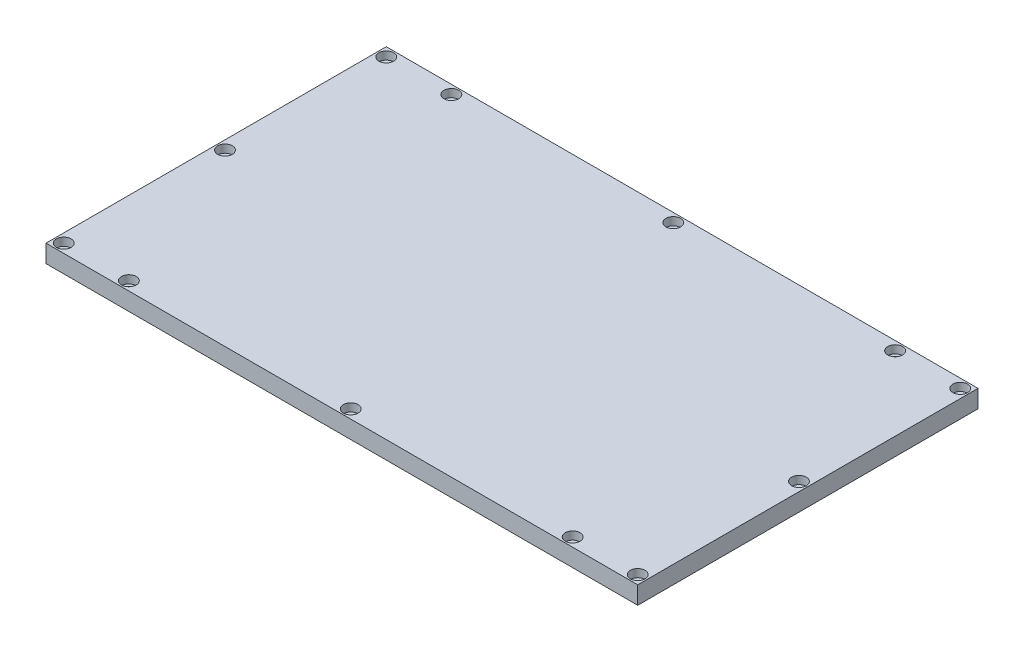
SolidWorks part; units mm, degrees
material "国产6061 "
ref_plane "Front Plane" through (0, 0, 0) normal (0, 0, 1) x (1, 0, 0)
ref_plane "Top Plane" through (0, 0, 0) normal (0, 1, 0) x (1, 0, 0)
ref_plane "Right Plane" through (0, 0, 0) normal (1, 0, 0) x (0, 0, -1)
sketch "Sketch1" plane through (0, 0, 0) normal (0, 1, 0) x (1, 0, 0)
  line L1 (-200, 115) -> (200, 115)
  line L2 (-200, 115) -> (-200, -115)
  line L3 (-200, -115) -> (200, -115)
  line L4 (200, 115) -> (200, -115)
  line L5 (-200, 115) -> (200, -115) construction
  line L6 (-200, -115) -> (200, 115) construction
  point P0 (0, 0)
  dimension "D1" = 400
  dimension "D2" = 230
extrude "Boss-Extrude1" add sketch "Sketch1" along normal blind 12
hole_wizard "CBORE for M5 Hex Socket Head Cap Screw1" positions "Sketch2" profile "Sketch3" counterbore size "M5" standard "ISO"
sketch "Sketch2" plane through (0, 12, 0) normal (0, 1, 0) x (1, 0, 0)
  line L0 (200, 115) -> (-200, 115) construction
  line L1 (-200, 115) -> (-200, -115) construction
  line L2 (-200, -115) -> (200, -115) construction
  line L3 (200, -115) -> (200, 115) construction
  point P0 (-194, 109)
  point P2 (-150, 109)
  point P4 (150, 109)
  point P6 (194, 109)
  point P8 (194, 0)
  point P10 (194, -109)
  point P12 (150, -109)
  point P14 (-150, -109)
  point P16 (-194, -109)
  point P18 (-194, 0)
  point P41 (0, 109)
  point P43 (0, -109)
  dimension "D1" = 6
  dimension "D2" = 6
  dimension "D3" = 6
  dimension "D4" = 6
  dimension "D5" = 150
  dimension "D6" = 150
sketch "Sketch3" plane through (-194, 12, -109) normal (1, 0, 0) x (0, 0, 1)
  line L0 (0, 0) -> (0, 26.1524)
  line L1 (0, 26.1524) -> (2.75, 24.5)
  line L2 (2.75, 24.5) -> (2.75, 5.4)
  line L3 (2.75, 5.4) -> (5, 5.4)
  line L4 (5, 5.4) -> (5, 0)
  line L5 (5, 0) -> (0, 0)
  line L10 (0, 26.1524) -> (-2.75, 24.5) construction
  line L11 (0, -6.35) -> (0, 107.95) construction
  dimension "孔直径" = 5.5
  dimension "孔深度" = 24.5
  dimension "柱形沉头孔直径" = 10
  dimension "柱形沉头孔深度" = 5.4
  dimension "导头角度" = 118
